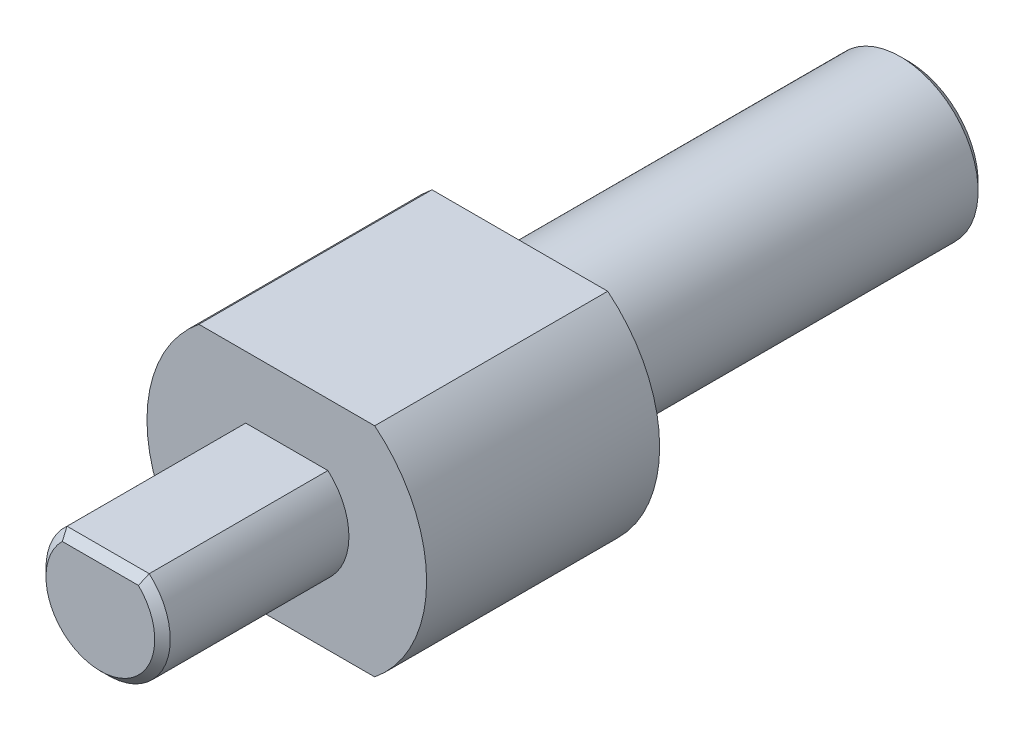
SolidWorks part; units mm, degrees
material "普通碳钢"
ref_plane "Front Plane" through (0, 0, 0) normal (0, 0, 1) x (1, 0, 0)
ref_plane "Top Plane" through (0, 0, 0) normal (0, 1, 0) x (1, 0, 0)
ref_plane "Right Plane" through (0, 0, 0) normal (1, 0, 0) x (0, 0, -1)
other "Configuration Table"
sketch "Sketch1" plane through (0, 0, 0) normal (0, 0, 1) x (1, 0, 0)
  line L0 (-2.6458, 3) -> (2.6458, 3)
  line L1 (0, 0) -> (0, 3) construction
  circle A0 centre (0, 0) radius 4
  dimension "D1" = 8
  dimension "D2" = 3
extrude "Boss-Extrude1" add sketch "Sketch1" against normal blind 12
sketch "Sketch2" plane through (0, 0, -12) normal (0, 0, -1) x (-1, 0, 0)
  line L1 (-5.6569, 7) -> (5.6569, 7)
  line L2 (0, 0) -> (12.3611, 0) construction
  line L4 (0, 0) -> (0, 7) construction
  line L5 (-5.6569, -7) -> (5.6569, -7)
  circle A2 centre (0, 0) radius 9
  arc M3 (-2.6458, 3) -> (2.6458, 3) centre (0, 0) ccw
  line M4 (2.6458, 3) -> (-2.6458, 3)
  dimension "D1" = 18
  dimension "D2" = 7
extrude "Boss-Extrude2" add sketch "Sketch2" along normal blind 15 contours L1 A2 L5 M3 M4 | M4 M3
sketch "Sketch3" plane through (0, 0, -27) normal (0, 0, -1) x (-1, 0, 0)
  circle A0 centre (0, 0) radius 5
  dimension "D1" = 10
extrude "Boss-Extrude3" add sketch "Sketch3" along normal blind 25
cosmetic thread "Cosmetic Thread1" parameters "D2"=8.376
chamfer "Chamfer1" distance 0.5 angle 45 3 edges at (0, 3, 0) (0, -4, 0) (-5, 0, -52)
